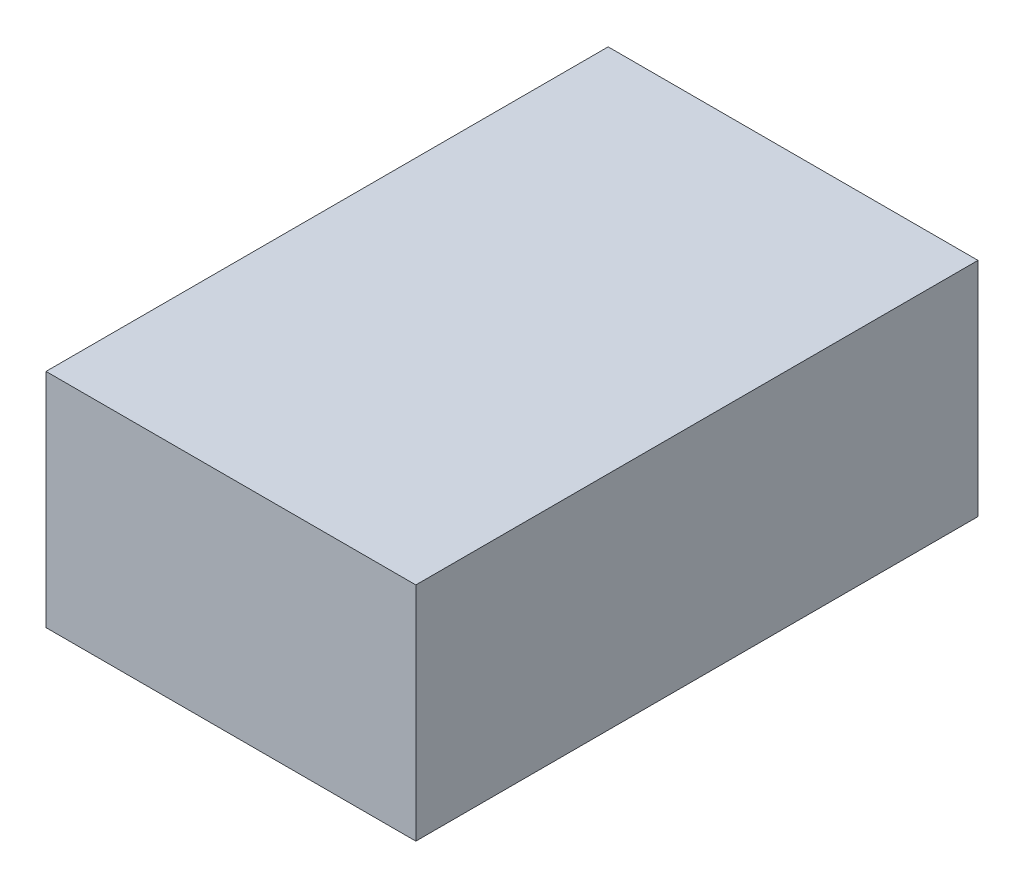
SolidWorks part; units mm, degrees
material "Q235A"
ref_plane "Front Plane" through (0, 0, 0) normal (0, 0, 1) x (1, 0, 0)
ref_plane "Top Plane" through (0, 0, 0) normal (0, 1, 0) x (1, 0, 0)
ref_plane "Right Plane" through (0, 0, 0) normal (1, 0, 0) x (0, 0, -1)
sketch "Sketch1" plane through (0, 0, 0) normal (0, 0, 1) x (1, 0, 0)
  line L1 (25, -15) -> (-25, -15)
  line L2 (25, -15) -> (25, 15)
  line L3 (25, 15) -> (-25, 15)
  line L4 (-25, -15) -> (-25, 15)
  line L5 (25, -15) -> (-25, 15) construction
  line L6 (25, 15) -> (-25, -15) construction
  point P0 (0, 0)
  dimension "D1" = 50
  dimension "D2" = 30
extrude "Boss-Extrude1" add sketch "Sketch1" along normal blind 76
